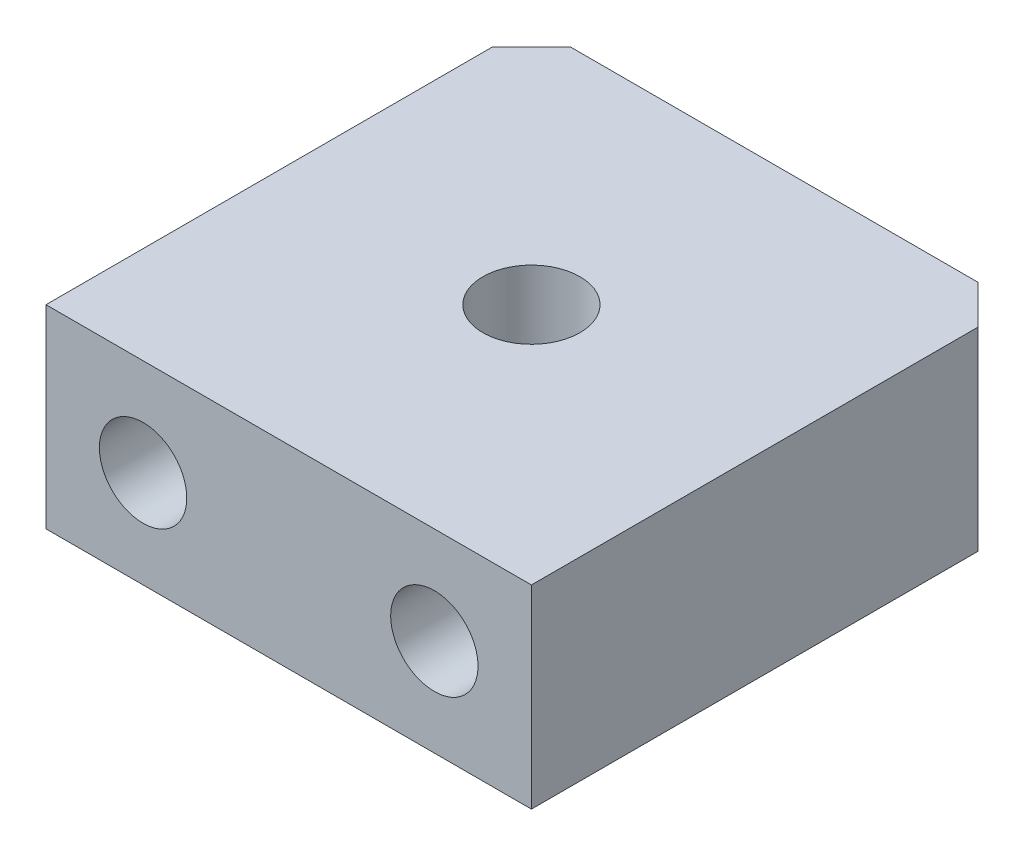
from build123d import *

# Parameters (mm, degrees)
SKETCH_1_W                   = 25
SKETCH_1_H                   = 25
EXTRUDE_1_DEPTH              = 10
CHAMFER_1_SIZE               = 2
HOLE_WIZARD_M6_1_D           = 5
HOLE_WIZARD_M4_1_D           = 4.5
HOLE_WIZARD_M4_1_CBORE_D     = 8
HOLE_WIZARD_M4_1_CBORE_DEPTH = 19.6


with BuildPart() as part:
    # 草图1 → 凸台-拉伸1 (new body)
    with BuildSketch(Plane(origin=(0, 0, 0), x_dir=(1, 0, 0), z_dir=(0, 1, 0))):
        Rectangle(SKETCH_1_W, SKETCH_1_H)
    extrude(amount=EXTRUDE_1_DEPTH)

    # 倒角1
    chamfer_1_edges = [part.edges().sort_by_distance(p)[0] for p in [
        (-12.5, 5, -12.5),
        (12.5, 5, -12.5),
    ]]
    chamfer(chamfer_1_edges, length=CHAMFER_1_SIZE)

    # M6 螺纹孔1 (through all)
    with Locations(Plane(origin=(0, 0, 0), x_dir=(-1, 0, 0), z_dir=(0, -1, 0))):
        with Locations((0, 0)):
            Hole(HOLE_WIZARD_M6_1_D / 2)

    # M4 六角圆柱头螺钉的柱形沉头孔1 (through all)
    with Locations(Plane(origin=(0, 0, -12.5), x_dir=(-1, 0, 0), z_dir=(0, 0, -1))):
        with Locations((-7.5, 5), (7.5, 5)):
            CounterBoreHole(HOLE_WIZARD_M4_1_D / 2, HOLE_WIZARD_M4_1_CBORE_D / 2, HOLE_WIZARD_M4_1_CBORE_DEPTH)


solid = part.part
